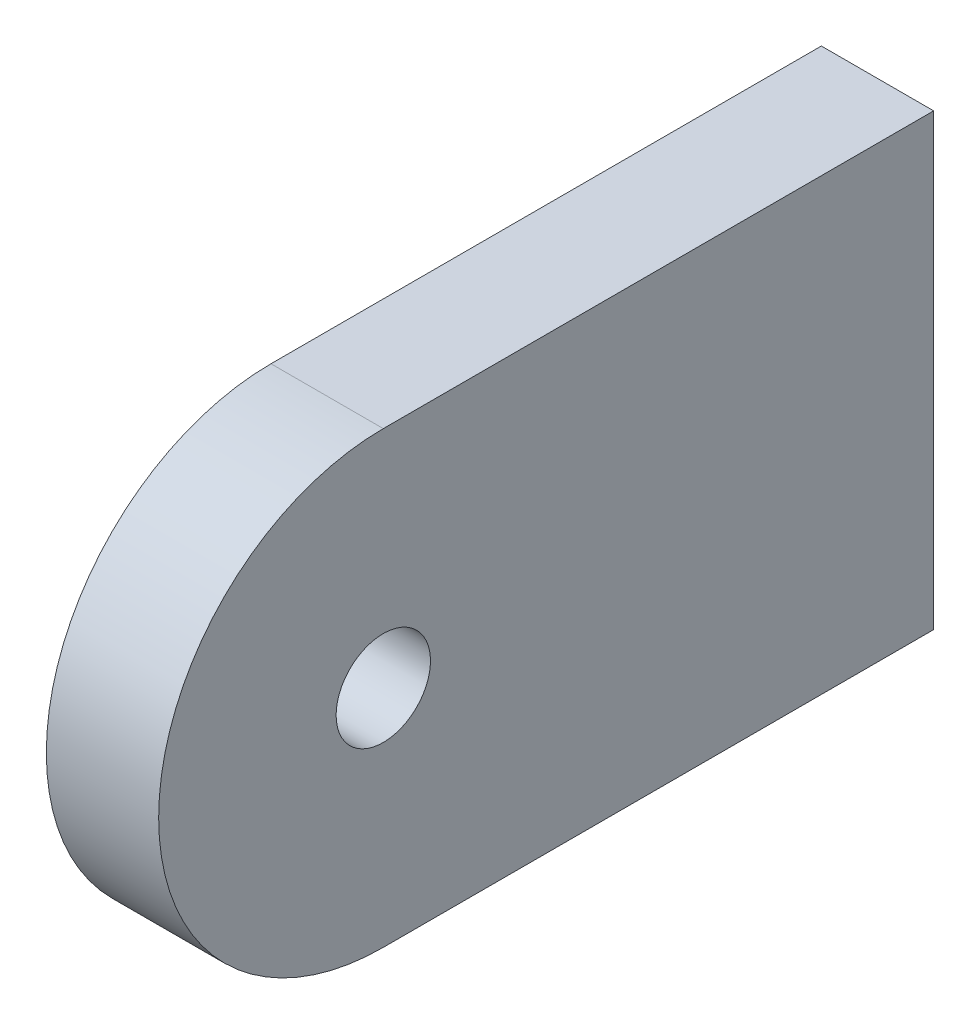
from build123d import *

# Parameters (mm, degrees)
BOSS_EXTRUDE1_DEPTH   = 2.5
M5_TAPPED_HOLE1_D     = 4.2
M5_TAPPED_HOLE1_DEPTH = 5
M5_TAPPED_HOLE1_TIP   = 1.2618073


with BuildPart() as part:
    # Sketch1 → Boss-Extrude1 (new, symmetric)
    with BuildSketch(Plane(origin=(0, 0, 0), x_dir=(0, 0, -1), z_dir=(1, 0, 0))):
        with BuildLine():
            Line((-15, 210), (-39.5, 210))
            ThreePointArc((-39.5, 210), (-49.5, 200), (-39.5, 190))
            Line((-39.5, 190), (-15, 190))
            Line((-15, 190), (-15, 210))
        make_face()
    extrude(amount=BOSS_EXTRUDE1_DEPTH, both=True)

    # M5 Tapped Hole1
    with Locations(Plane(origin=(-2.5, 200, 39.5), x_dir=(0, 0, -1), z_dir=(-1, 0, 0))):
        with Locations((0, 0)):
            Hole(M5_TAPPED_HOLE1_D / 2, depth=M5_TAPPED_HOLE1_DEPTH)
            with Locations((0, 0, -(M5_TAPPED_HOLE1_DEPTH + M5_TAPPED_HOLE1_TIP / 2))):  # 118° drill point
                Cone(0, M5_TAPPED_HOLE1_D / 2, M5_TAPPED_HOLE1_TIP, mode=Mode.SUBTRACT)


solid = part.part
